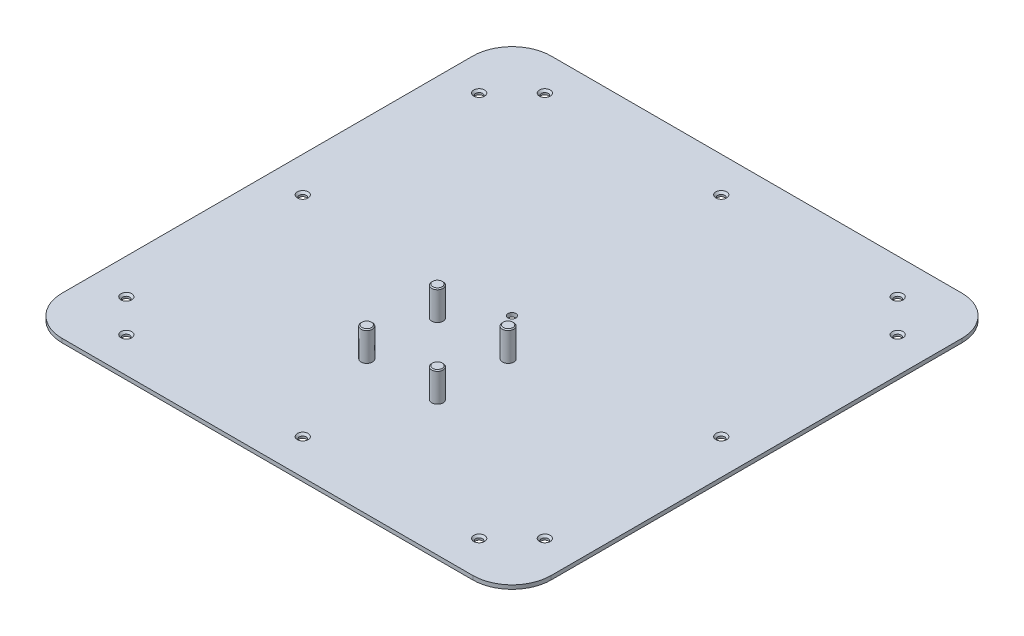
from build123d import *

# Parameters (mm, degrees)
SKETCH1_R           = 1.75
SKETCH1_R_2         = 2
BOSS_EXTRUDE1_DEPTH = 2
CHAMFER1_SIZE       = 1
SKETCH3_R           = 2.9
BOSS_EXTRUDE2_DEPTH = 15
CHAMFER2_SIZE       = 0.5


with BuildPart() as part:
    # Sketch1 → Boss-Extrude1 (new body)
    with BuildSketch(Plane(origin=(0, 0, 0), x_dir=(1, 0, 0), z_dir=(0, 1, 0))):
        with BuildLine():
            Line((-104.75, -124.75), (104.75, -124.75))
            ThreePointArc((104.75, -124.75), (118.892135624, -118.892135624), (124.75, -104.75))
            Line((124.75, -104.75), (124.75, 104.75))
            ThreePointArc((124.75, 104.75), (118.892135624, 118.892135624), (104.75, 124.75))
            Line((104.75, 124.75), (-104.75, 124.75))
            ThreePointArc((-104.75, 124.75), (-118.892135624, 118.892135624), (-124.75, 104.75))
            Line((-124.75, 104.75), (-124.75, -104.75))
            ThreePointArc((-124.75, -104.75), (-118.892135624, -118.892135624), (-104.75, -124.75))
        make_face()
        with Locations(Location((-90, 106.75, 0), (0, 0, 270))):
            Circle(SKETCH1_R, mode=Mode.SUBTRACT)
        with Locations(Location((0, 106.75, 0), (0, 0, 270))):
            Circle(SKETCH1_R, mode=Mode.SUBTRACT)
        with Locations(Location((90, 106.75, 0), (0, 0, 270))):
            Circle(SKETCH1_R, mode=Mode.SUBTRACT)
        with Locations(Location((106.75, 90, 0), (0, 0, 270))):
            Circle(SKETCH1_R, mode=Mode.SUBTRACT)
        with Locations(Location((106.75, 0, 0), (0, 0, 270))):
            Circle(SKETCH1_R, mode=Mode.SUBTRACT)
        with Locations(Location((106.75, -90, 0), (0, 0, 270))):
            Circle(SKETCH1_R, mode=Mode.SUBTRACT)
        with Locations(Location((90, -106.75, 0), (0, 0, 270))):
            Circle(SKETCH1_R, mode=Mode.SUBTRACT)
        with Locations(Location((0, -106.75, 0), (0, 0, 270))):
            Circle(SKETCH1_R, mode=Mode.SUBTRACT)
        with Locations(Location((-90, -106.75, 0), (0, 0, 270))):
            Circle(SKETCH1_R, mode=Mode.SUBTRACT)
        with Locations(Location((-106.75, -90, 0), (0, 0, 270))):
            Circle(SKETCH1_R, mode=Mode.SUBTRACT)
        with Locations(Location((-106.75, 0, 0), (0, 0, 270))):
            Circle(SKETCH1_R, mode=Mode.SUBTRACT)
        with Locations(Location((-106.75, 90, 0), (0, 0, 270))):
            Circle(SKETCH1_R, mode=Mode.SUBTRACT)
        with Locations(Location((0, 0, 0), (0, 0, 270))):
            Circle(SKETCH1_R_2, mode=Mode.SUBTRACT)
    extrude(amount=BOSS_EXTRUDE1_DEPTH)

    # Chamfer1
    chamfer1_edges = [part.edges().sort_by_distance(p)[0] for p in [
        (-90, 2, -108.5),
        (0, 2, -108.5),
        (90, 2, -108.5),
        (106.75, 2, -91.75),
        (106.75, 2, -1.75),
        (106.75, 2, 88.25),
        (90, 2, 105),
        (0, 2, 105),
        (-90, 2, 105),
        (-106.75, 2, 88.25),
        (-106.75, 2, -1.75),
        (-106.75, 2, -91.75),
    ]]
    chamfer(chamfer1_edges, length=CHAMFER1_SIZE)

    # Sketch3 → Boss-Extrude2 (add)
    with BuildSketch(Plane(origin=(0, 2, 0), x_dir=(1, 0, 0), z_dir=(0, 1, 0))):
        with Locations(Location((-18.03122292, -20, 0), (0, 0, 90))):
            Circle(SKETCH3_R)
        with Locations(Location((18.03122292, -20, 0), (0, 0, 90))):
            Circle(SKETCH3_R)
        with Locations(Location((18.03122292, -56.062445841, 0), (0, 0, 90))):
            Circle(SKETCH3_R)
        with Locations(Location((-18.03122292, -56.062445841, 0), (0, 0, 90))):
            Circle(SKETCH3_R)
    extrude(amount=BOSS_EXTRUDE2_DEPTH)

    # Chamfer2
    chamfer2_edges = [part.edges().sort_by_distance(p)[0] for p in [
        (-18.03122292, 17, 22.9),
        (18.03122292, 17, 22.9),
        (18.03122292, 17, 58.962445841),
        (-18.03122292, 17, 58.962445841),
    ]]
    chamfer(chamfer2_edges, length=CHAMFER2_SIZE)


solid = part.part
